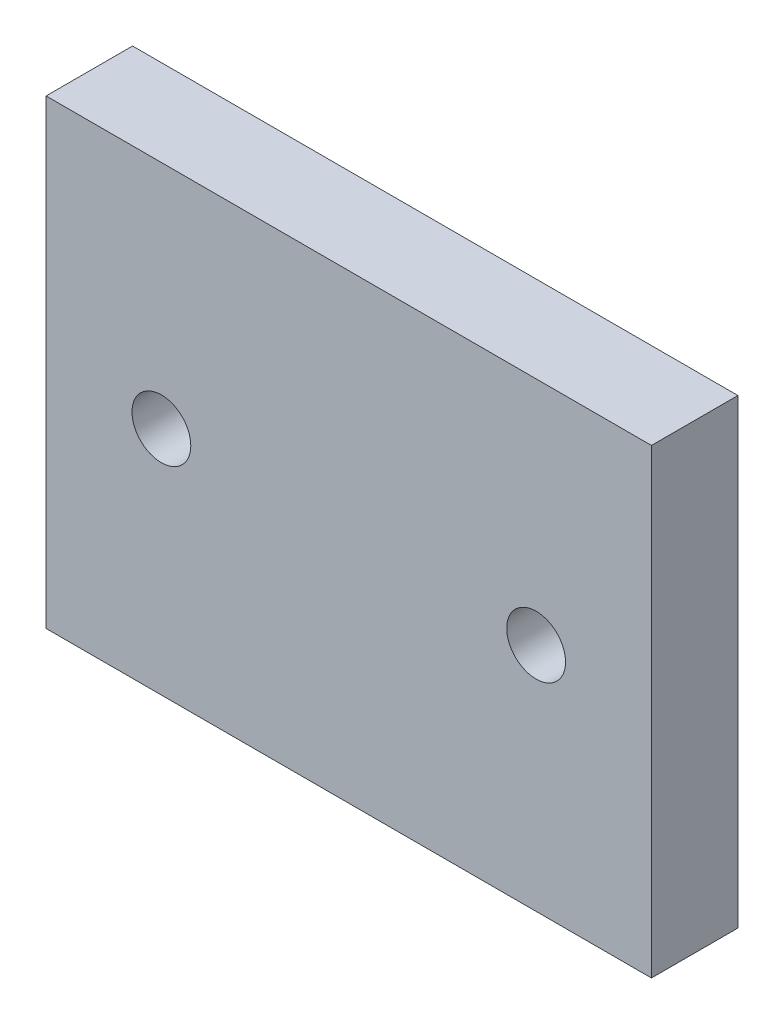
from build123d import *

# Parameters (mm, degrees)
SKETCH_1_W              = 105
SKETCH_1_H              = 80
EXTRUDE_1_DEPTH         = 15
HOLE_WIZARD_M12_1_D     = 10.2
HOLE_WIZARD_M12_1_DEPTH = 29.25
HOLE_WIZARD_M12_1_TIP   = 3.064389157


with BuildPart() as part:
    # 草图1 → 凸台-拉伸1 (new body)
    with BuildSketch(Plane.XY):
        Rectangle(SKETCH_1_W, SKETCH_1_H)
    extrude(amount=EXTRUDE_1_DEPTH)

    # M12 螺纹孔1
    with Locations(Plane.XY.offset(15)):
        with Locations((-32.5, 0), (32.5, 0)):
            Hole(HOLE_WIZARD_M12_1_D / 2, depth=HOLE_WIZARD_M12_1_DEPTH)
            with Locations((0, 0, -(HOLE_WIZARD_M12_1_DEPTH + HOLE_WIZARD_M12_1_TIP / 2))):  # 118° drill point
                Cone(0, HOLE_WIZARD_M12_1_D / 2, HOLE_WIZARD_M12_1_TIP, mode=Mode.SUBTRACT)


solid = part.part
